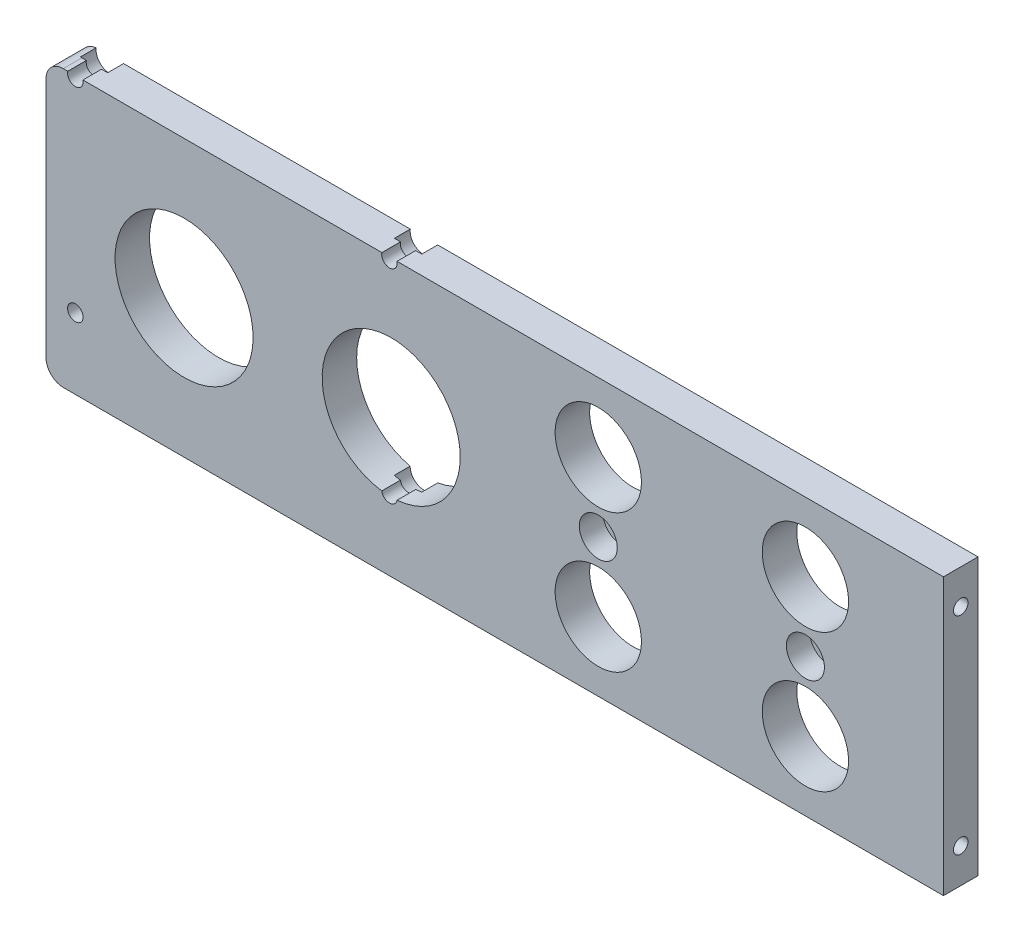
SolidWorks part; units mm, degrees
ref_plane "前视基准面" through (0, 0, 0) normal (0, 0, 1) x (1, 0, 0)
ref_plane "上视基准面" through (0, 0, 0) normal (0, 1, 0) x (1, 0, 0)
ref_plane "右视基准面" through (0, 0, 0) normal (1, 0, 0) x (0, 0, -1)
sketch "草图1" plane through (0, 0, 0) normal (0, 0, 1) x (1, 0, 0)
  line L1 (130, -40) -> (-130, -40)
  line L2 (130, -40) -> (130, 40)
  line L3 (130, 40) -> (-130, 40)
  line L4 (-130, -40) -> (-130, 40)
  line L5 (130, -40) -> (-130, 40) construction
  line L6 (130, 40) -> (-130, -40) construction
  point P0 (0, 0)
  dimension "D1" = 80
  dimension "D2" = 260
extrude "凸台-拉伸1" add sketch "草图1" along normal blind 10
sketch "草图2" plane through (0, 0, 10) normal (0, 0, 1) x (1, 0, 0)
  line L0 (-130, 0) -> (-90, 0) construction
  line L1 (-130, 40) -> (-130, -40) construction
  line L2 (-90, 0) -> (-30, 0) construction
  circle A0 centre (-90, 0) radius 20
  circle A1 centre (-30, 0) radius 20
  dimension "D2" = 40
  dimension "D1" = 40
  dimension "D3" = 60
extrude "切除-拉伸1" cut sketch "草图2" against normal up to next
sketch "草图3" plane through (0, 0, 10) normal (0, 0, 1) x (1, 0, 0)
  line L0 (30, -20) -> (30, 20) construction
  line L1 (30, 20) -> (90, 20) construction
  line L2 (90, 20) -> (90, -20) construction
  line L3 (90, -20) -> (30, -20) construction
  line L4 (90, 0) -> (130, 0) construction
  line L5 (130, -40) -> (130, 40) construction
  circle A0 centre (30, -20) radius 12.5
  circle A1 centre (90, -20) radius 12.5
  circle A2 centre (30, 20) radius 12.5
  circle A3 centre (90, 20) radius 12.5
  dimension "D2" = 25
  dimension "D1" = 40
  dimension "D3" = 40
  dimension "D4" = 60
extrude "切除-拉伸2" cut sketch "草图3" against normal up to next
hole_wizard "M5 螺纹孔1" positions "草图4" profile "草图6" tap size "M5" standard "GB"
sketch "草图4" plane through (130, 0, 0) normal (1, 0, 0) x (0, 0, -1)
  line L0 (-5, 30) -> (-5, -30) construction
  line L1 (-5, -30) -> (-5, -40) construction
  line L2 (-10, -40) -> (0, -40) construction
  line L5 (0, 0) -> (-5, 0) construction
  point P0 (-5, 30)
  point P2 (-5, -30)
  dimension "D1" = 60
sketch "草图6" plane through (130, 30, 5) normal (0, 1, 0) x (0, 0, -1)
  line L0 (0, 0) -> (0, 13.6618)
  line L1 (0, 13.6618) -> (2.1, 12.4)
  line L2 (2.1, 12.4) -> (2.1, 0)
  line L5 (2.1, 0) -> (0, 0)
  line L10 (0, 13.6618) -> (-2.1, 12.4) construction
  line L11 (0, -6.35) -> (0, 107.95) construction
  dimension "螺纹孔钻头直径" = 4.2
  dimension "螺纹孔钻头深度" = 12.4
  dimension "导头角度" = 118
cosmetic thread "孔螺蚊线1" parameters "D1"=10, "D2"=5
cosmetic thread "孔螺蚊线2" parameters "D1"=10, "D2"=5
hole_wizard "打孔尺寸(%根据)内六角圆柱头螺钉的类型1" positions "草图7" profile "草图8" counterbore size "M6" standard "GB" end condition up to next
sketch "草图7" plane through (0, 0, 10) normal (0, 0, 1) x (1, 0, 0)
  point P0 (90, 0)
  point P3 (30, 0)
sketch "草图8" plane through (90, 0, 10) normal (1, 0, 0) x (0, -1, 0)
  line L0 (0, 0) -> (0, 10)
  line L1 (0, 10) -> (3.3, 10)
  line L3 (3.3, 10) -> (3.3, 6.8)
  line L4 (3.3, 6.8) -> (5.5, 6.8)
  line L5 (5.5, 6.8) -> (5.5, 0)
  line L7 (5.5, 0) -> (0, 0)
  line L11 (0, -6.35) -> (0, 107.95) construction
  dimension "通孔孔直径" = 6.6
  dimension "通孔孔深度" = 10
  dimension "柱形沉头孔直径" = 11
  dimension "柱形沉头孔深度" = 6.8
hole_wizard "打孔尺寸(%根据)内六角圆柱头螺钉的类型2" positions "草图9" profile "草图10" counterbore size "M4" standard "GB" end condition up to next
sketch "草图9" plane through (0, 0, 0) normal (0, 0, -1) x (-1, 0, 0)
  point P0 (30.5, -19.5)
  point P3 (30.5, 39.5)
  point P6 (121.5, 39.5)
  point P9 (121.5, -19.5)
sketch "草图10" plane through (-30.5, -19.5, 0) normal (1, 0, 0) x (0, 1, 0)
  line L0 (0, 0) -> (0, 10)
  line L1 (0, 10) -> (2.25, 10)
  line L3 (2.25, 10) -> (2.25, 4.6)
  line L4 (2.25, 4.6) -> (4, 4.6)
  line L5 (4, 4.6) -> (4, 0)
  line L7 (4, 0) -> (0, 0)
  line L11 (0, -6.35) -> (0, 107.95) construction
  dimension "通孔孔直径" = 4.5
  dimension "通孔孔深度" = 10
  dimension "柱形沉头孔直径" = 8
  dimension "柱形沉头孔深度" = 4.6
fillet "圆角1" radius 5 2 edges at (-130, 40, 5) (-130, -40, 5)
